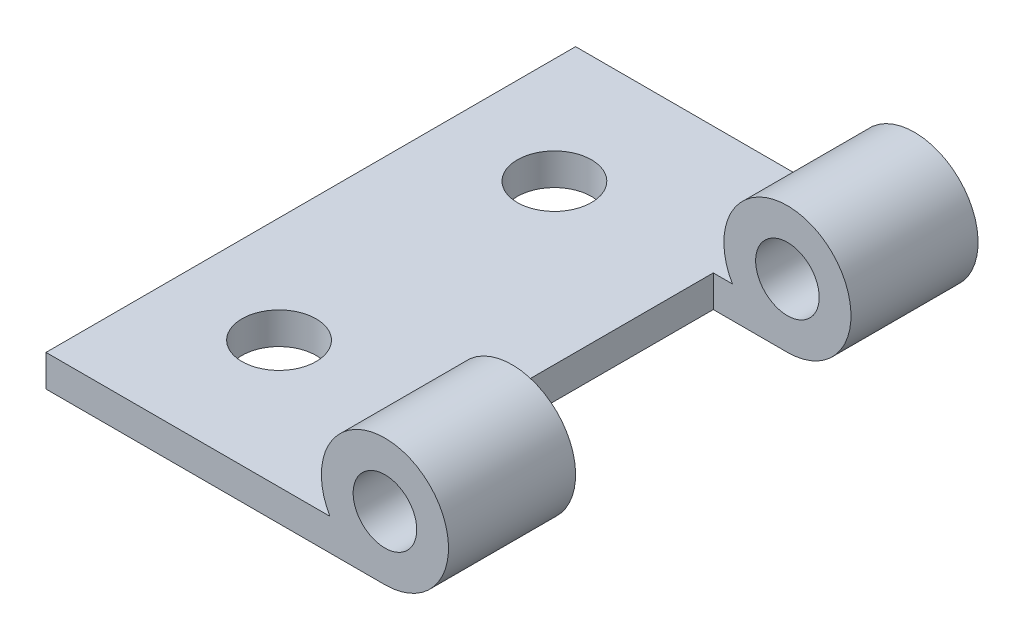
from build123d import *

# Parameters (mm, degrees)
SKETCH_1_R          = 1.5
EXTRUDE_1_DEPTH     = 12.5
CUT_EXTRUDE_1_DEPTH = 6.5
SKETCH_3_R          = 1.75
CUT_EXTRUDE_2_DEPTH = 21.796634343


with BuildPart() as part:
    # 草图1 → 凸台-拉伸1 (new, symmetric)
    with BuildSketch(Plane.XY):
        with BuildLine():
            Line((-2.598076211, -1.5), (-16, -1.5))
            Line((-16, -1.5), (-16, -3))
            Line((-16, -3), (0, -3))
            ThreePointArc((0, -3), (1.5, 2.598076211), (-2.598076211, -1.5))
        make_face()
        Circle(SKETCH_1_R, mode=Mode.SUBTRACT)
    extrude(amount=EXTRUDE_1_DEPTH, both=True)

    # 草图2 → 切除-拉伸1 (cut, symmetric)
    with BuildSketch(Plane.XY):
        with BuildLine():
            Line((-3.5, 0), (-3.5, -3))
            Line((-3.5, -3), (-1.802775638, -3))
            ThreePointArc((-1.802775638, -3), (3.046285831, 1.723410176), (-3.5, 0))
        make_face()
    extrude(amount=CUT_EXTRUDE_1_DEPTH, both=True, mode=Mode.SUBTRACT)

    # 草图3 → 切除-拉伸2 (cut, through all)
    with BuildSketch(Plane(origin=(0, -1.5, 0), x_dir=(1, 0, 0), z_dir=(0, 1, 0))):
        with Locations(Location((-11, 6.5, 0), (0, 0, 180))):
            Circle(SKETCH_3_R)
        with Locations((-11, -6.5)):
            Circle(SKETCH_3_R)
    extrude(amount=-CUT_EXTRUDE_2_DEPTH, mode=Mode.SUBTRACT)


solid = part.part
